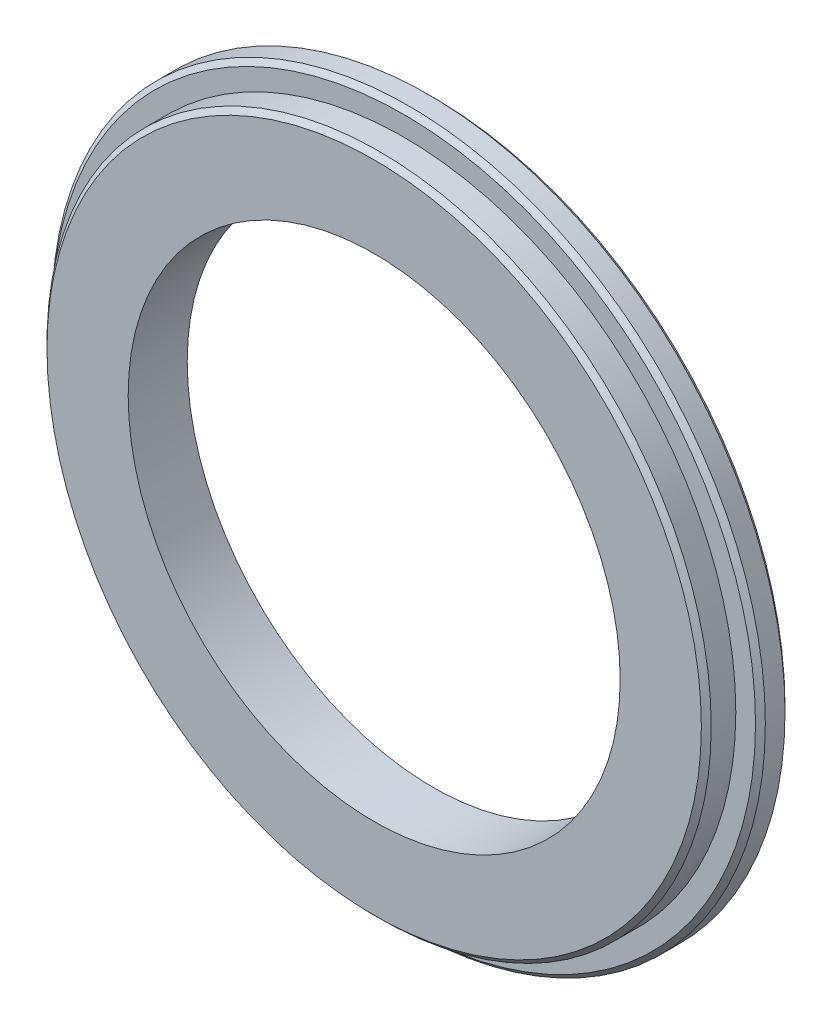
from build123d import *

# Parameters (mm, degrees)
SKETCH1_R             = 72.5
SKETCH1_R_2           = 50
BOSS_EXTRUDE1_DEPTH   = 6
SKETCH2_R             = 67.5
SKETCH2_R_2           = 50
BOSS_EXTRUDE2_DEPTH   = 6
CHAMFER1_SIZE         = 1
SKETCH3_R             = 3
CUT_EXTRUDE1_DEPTH    = 8
M8_TAPPED_HOLE1_D     = 6.8
M8_TAPPED_HOLE1_DEPTH = 8
M8_TAPPED_HOLE1_TIP   = 2.042926105


with BuildPart() as part:
    # Sketch1 → Boss-Extrude1 (new body)
    with BuildSketch(Plane.XY):
        Circle(SKETCH1_R)
        Circle(SKETCH1_R_2, mode=Mode.SUBTRACT)
    extrude(amount=BOSS_EXTRUDE1_DEPTH)

    # Sketch2 → Boss-Extrude2 (add)
    with BuildSketch(Plane.XY.offset(6)):
        Circle(SKETCH2_R)
        Circle(SKETCH2_R_2, mode=Mode.SUBTRACT)
    extrude(amount=BOSS_EXTRUDE2_DEPTH)

    # Chamfer1
    chamfer1_edges = [part.edges().sort_by_distance(p)[0] for p in [
        (-67.5, 0, 12),
        (-72.5, 0, 0),
        (-72.5, 0, 6),
    ]]
    chamfer(chamfer1_edges, length=CHAMFER1_SIZE)

    # Sketch3 → Cut-Extrude1 (cut)
    with BuildSketch(Plane(origin=(0, 0, 0), x_dir=(-1, 0, 0), z_dir=(0, 0, -1))):
        with Locations((-30, 51.961524227)):
            Circle(SKETCH3_R)
        with Locations((-60, 0)):
            Circle(SKETCH3_R)
        with Locations((30, 51.961524227)):
            Circle(SKETCH3_R)
        with Locations((60, 0)):
            Circle(SKETCH3_R)
        with Locations((30, -51.961524227)):
            Circle(SKETCH3_R)
        with Locations((-30, -51.961524227)):
            Circle(SKETCH3_R)
    extrude(amount=-CUT_EXTRUDE1_DEPTH, mode=Mode.SUBTRACT)

    # M8 Tapped Hole1
    with Locations(Plane(origin=(0, 0, 0), x_dir=(-1, 0, 0), z_dir=(0, 0, -1))):
        with Locations((-30, 51.961524227), (30, 51.961524227), (60, 0), (30, -51.961524227), (-30, -51.961524227), (-60, 0)):
            Hole(M8_TAPPED_HOLE1_D / 2, depth=M8_TAPPED_HOLE1_DEPTH)
            with Locations((0, 0, -(M8_TAPPED_HOLE1_DEPTH + M8_TAPPED_HOLE1_TIP / 2))):  # 118° drill point
                Cone(0, M8_TAPPED_HOLE1_D / 2, M8_TAPPED_HOLE1_TIP, mode=Mode.SUBTRACT)


solid = part.part
